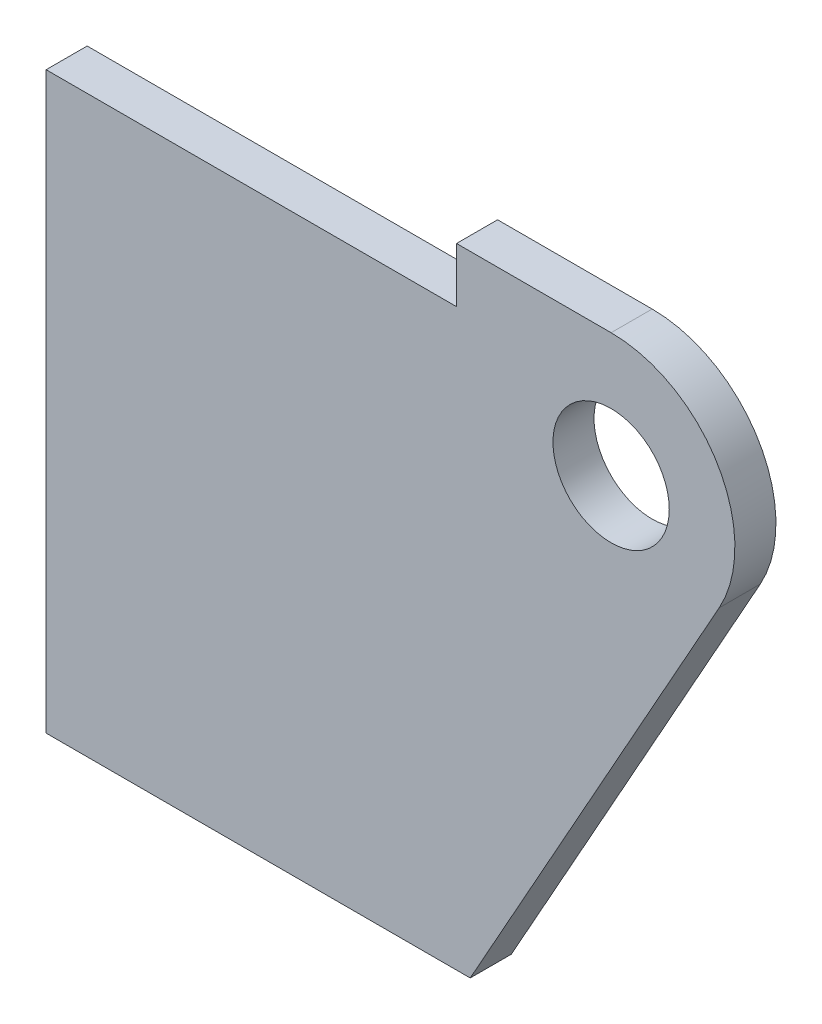
SolidWorks part; units mm, degrees
ref_plane "Front Plane" through (0, 0, 0) normal (0, 0, 1) x (1, 0, 0)
ref_plane "Top Plane" through (0, 0, 0) normal (0, 1, 0) x (1, 0, 0)
ref_plane "Right Plane" through (0, 0, 0) normal (1, 0, 0) x (0, 0, -1)
sketch "Sketch1" plane through (0, 0, 0) normal (0, 0, 1) x (1, 0, 0)
  line L0 (0, 0) -> (0, 420)
  line L1 (300, 460) -> (413, 460)
  line L2 (0, 0) -> (310, 0)
  line L3 (310, 0) -> (491.9821, 325.3176)
  line L4 (0, 420) -> (300, 420)
  line L5 (300, 420) -> (300, 460)
  arc A0 (491.9821, 325.3176) -> (413, 460) centre (413, 369.5) ccw
  circle A1 centre (413, 369.5) radius 42.5
  dimension "D6" = 85
  dimension "D1" = 460
  dimension "D2" = 310
  dimension "D3" = 413
  dimension "D4" = 90.5
  dimension "D5" = 0
  dimension "D7" = 40
  dimension "D8" = 300
extrude "Boss-Extrude1" add sketch "Sketch1" along normal blind 30
